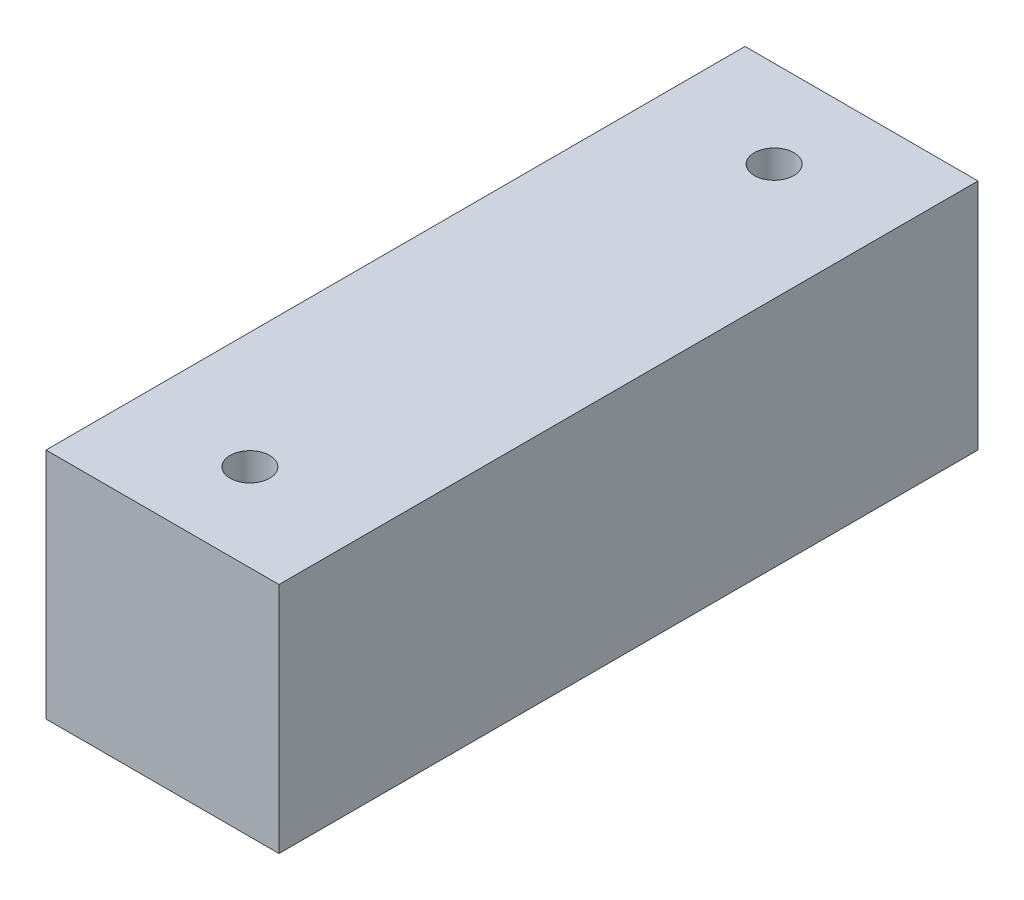
SolidWorks part; units mm, degrees
material "1023 碳钢板 (SS)"
ref_plane "Front Plane" through (0, 0, 0) normal (0, 0, 1) x (1, 0, 0)
ref_plane "Top Plane" through (0, 0, 0) normal (0, 1, 0) x (1, 0, 0)
ref_plane "Right Plane" through (0, 0, 0) normal (1, 0, 0) x (0, 0, -1)
sketch "Sketch1" plane through (0, 0, 0) normal (0, 0, 1) x (1, 0, 0)
  line L1 (30, 30) -> (-30, 30)
  line L2 (30, 30) -> (30, -30)
  line L3 (30, -30) -> (-30, -30)
  line L4 (-30, 30) -> (-30, -30)
  line L5 (30, 30) -> (-30, -30) construction
  line L6 (30, -30) -> (-30, 30) construction
  point P0 (0, 0)
  dimension "D1" = 60
  dimension "D2" = 60
extrude "Boss-Extrude1" add sketch "Sketch1" along normal blind 180
sketch "Sketch2" plane through (0, 30, 0) normal (0, 1, 0) x (1, 0, 0)
  line L0 (30, -180) -> (-30, -180) construction
  circle A0 centre (0, -22.5) radius 13.968
  circle A1 centre (0, -157.5) radius 13.5734
  dimension "D1" = 135
  dimension "D2" = 22.5
hole_wizard "M12 Tapped Hole1" positions "Sketch3" profile "Sketch4" tap size "M12" standard "ISO" end condition through all
sketch "Sketch3" plane through (0, 30, 0) normal (0, 1, 0) x (1, 0, 0)
  point P0 (0, -22.5)
  point P3 (0, -157.5)
cosmetic thread "Hole thread line 1"
cosmetic thread "Hole thread line 2"
sketch "Sketch4" plane through (0, 30, 22.5) normal (1, 0, 0) x (0, 0, 1)
  line L0 (0, 0) -> (0, 60)
  line L1 (0, 60) -> (5.1, 60)
  line L2 (5.1, 60) -> (5.1, 0)
  line L5 (5.1, 0) -> (0, 0)
  line L11 (0, -6.35) -> (0, 107.95) construction
  dimension "通孔螺纹孔钻头直径" = 10.2
  dimension "通孔螺纹孔钻头深度" = 60
